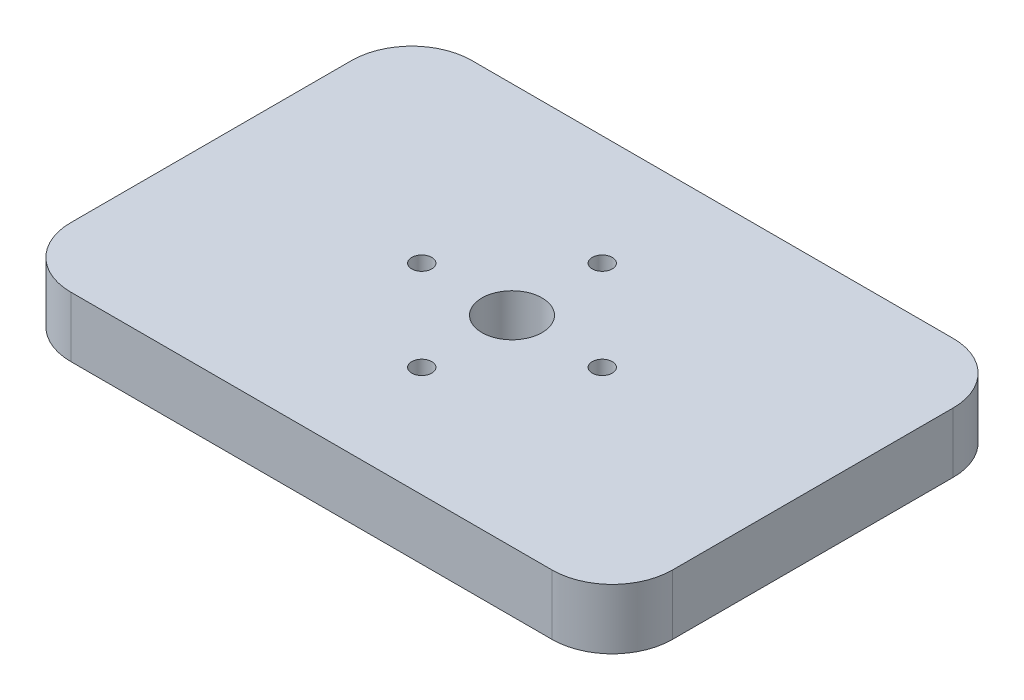
from build123d import *

# Parameters (mm, degrees)
SKETCH1_W           = 300
SKETCH1_H           = 200
BOSS_EXTRUDE1_DEPTH = 30
SKETCH2_R           = 15
SKETCH2_R_2         = 5
CUT_EXTRUDE1_DEPTH  = 30
FILLET1_R           = 30


with BuildPart() as part:
    # Sketch1 → Boss-Extrude1 (new body)
    with BuildSketch(Plane(origin=(0, 0, 0), x_dir=(1, 0, 0), z_dir=(0, 1, 0))):
        Rectangle(SKETCH1_W, SKETCH1_H)
    extrude(amount=BOSS_EXTRUDE1_DEPTH)

    # Sketch2 → Cut-Extrude1 (cut)
    with BuildSketch(Plane(origin=(0, 30, 0), x_dir=(1, 0, 0), z_dir=(0, 1, 0))):
        with Locations(Location((0, 0, 0), (0, 0, 270))):
            Circle(SKETCH2_R)
        with Locations(Location((0, 45, 0), (0, 0, 270))):
            Circle(SKETCH2_R_2)
        with Locations(Location((-45, 0, 0), (0, 0, 270))):
            Circle(SKETCH2_R_2)
        with Locations(Location((0, -45, 0), (0, 0, 90))):
            Circle(SKETCH2_R_2)
        with Locations(Location((45, 0, 0), (0, 0, 90))):
            Circle(SKETCH2_R_2)
    extrude(amount=-CUT_EXTRUDE1_DEPTH, mode=Mode.SUBTRACT)

    # Fillet1
    fillet1_edges = [part.edges().sort_by_distance(p)[0] for p in [
        (150, 15, 100),
        (-150, 15, 100),
        (-150, 15, -100),
        (150, 15, -100),
    ]]
    fillet(fillet1_edges, radius=FILLET1_R)


solid = part.part
